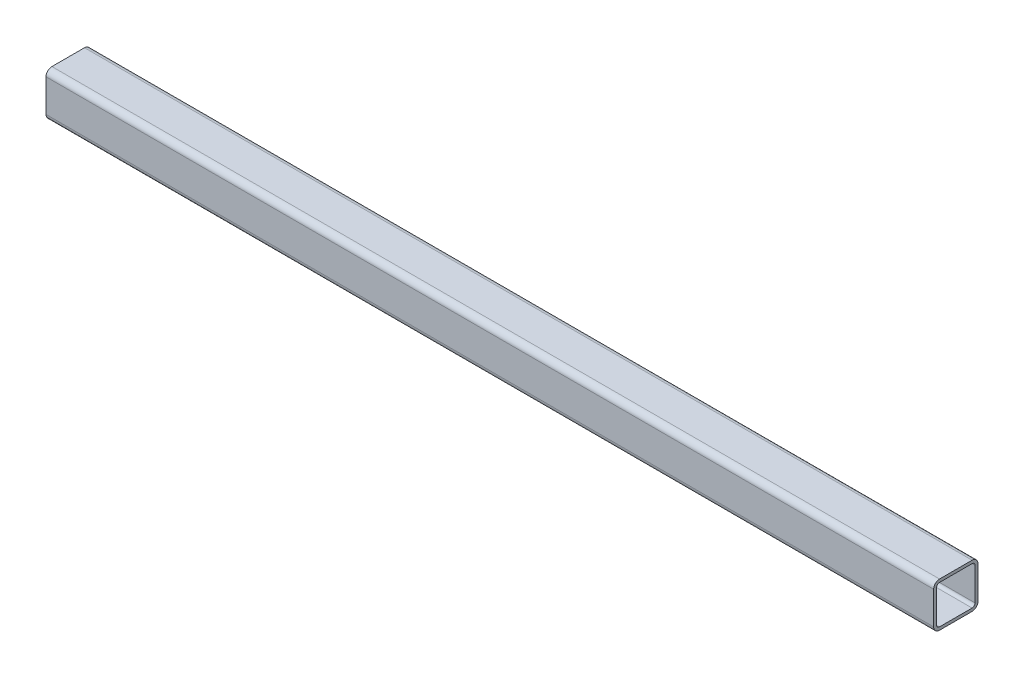
SolidWorks part; units mm, degrees
ref_plane "前视基准面" through (0, 0, 0) normal (0, 0, 1) x (1, 0, 0)
ref_plane "上视基准面" through (0, 0, 0) normal (0, 1, 0) x (1, 0, 0)
ref_plane "右视基准面" through (0, 0, 0) normal (1, 0, 0) x (0, 0, -1)
sketch "草图1" plane through (0, 0, 0) normal (0, 1, 0) x (1, 0, 0)
  line L0 (-600, 0) -> (600, 0)
  line L1 (-605, 0) -> (605, 0) construction
  point P5 (0, 0)
  dimension "D1" = 1200
other "Gb／6728-1986方形空心型钢 60 X 60 X 4(1)"
ref_plane "基准面1" through (-600, 0, 0) normal (1, 0, 0) x (0, 0, -1)
sketch "Sketch11" plane through (-600, 0, 0) normal (1, 0, 0) x (0, 0, -1)
  line L0 (-22, -26) -> (22, -26)
  line L1 (-26, -22) -> (-26, 22)
  line L2 (22, 26) -> (-22, 26)
  line L3 (26, 22) -> (26, -22)
  line L4 (-22, -30) -> (22, -30)
  line L5 (-30, -22) -> (-30, 22)
  line L6 (22, 30) -> (-22, 30)
  line L7 (30, 22) -> (30, -22)
  arc A0 (30, 22) -> (22, 30) centre (22, 22) ccw
  arc A1 (22, -30) -> (30, -22) centre (22, -22) ccw
  arc A2 (-30, -22) -> (-22, -30) centre (-22, -22) ccw
  arc A3 (-22, 30) -> (-30, 22) centre (-22, 22) ccw
  arc A4 (-22, 26) -> (-26, 22) centre (-22, 22) ccw
  arc A5 (26, 22) -> (22, 26) centre (22, 22) ccw
  arc A6 (22, -26) -> (26, -22) centre (22, -22) ccw
  arc A7 (-26, -22) -> (-22, -26) centre (-22, -22) ccw
  point P0 (-30, 0)
  point P1 (30, 0)
  point P2 (0, 30)
  point P3 (0, -30)
  point P4 (0, 0)
  point P5 (-30, -30)
  point P6 (30, -30)
  point P7 (30, 30)
  point P8 (-30, 30)
  point P33 (0, 0)
  dimension "D1" = 8
  dimension "Thickness" = 4
  dimension "V_leg" = 60
